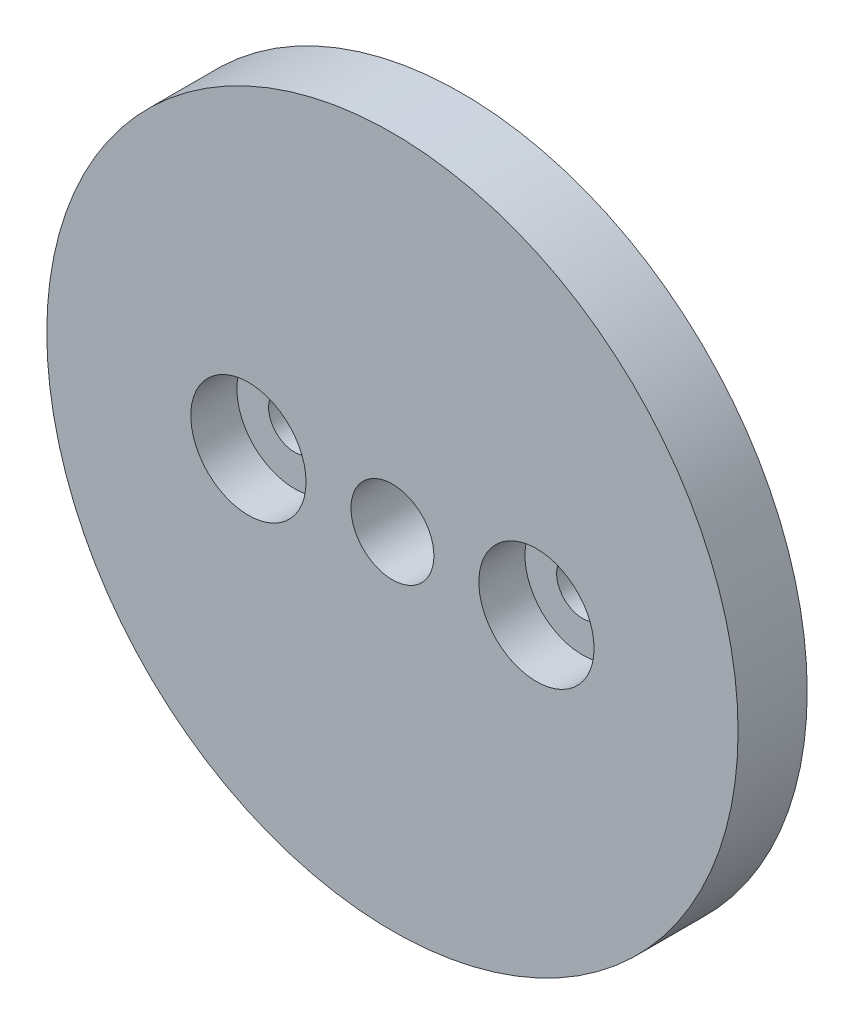
SolidWorks part; units mm, degrees
ref_plane "Front Plane" through (0, 0, 0) normal (0, 0, 1) x (1, 0, 0)
ref_plane "Top Plane" through (0, 0, 0) normal (0, 1, 0) x (1, 0, 0)
ref_plane "Right Plane" through (0, 0, 0) normal (1, 0, 0) x (0, 0, -1)
sketch "Sketch1" plane through (0, 0, 0) normal (0, 0, 1) x (1, 0, 0)
  circle A0 centre (0, 0) radius 30
  dimension "D1" = 60
extrude "Boss-Extrude1" add sketch "Sketch1" along normal blind 6
hole_wizard "CBORE for M4 Hex Head Bolt1" positions "Sketch2" profile "Sketch3" counterbore size "M4" standard "GB" end condition through all
sketch "Sketch2" plane through (0, 0, 6) normal (0, 0, 1) x (1, 0, 0)
  line L0 (0, 0) -> (0, 26.9917) construction
  point P0 (-12.5, 0)
  point P8 (12.5, 0)
  dimension "D1" = 12.5
sketch "Sketch3" plane through (-12.5, 0, 6) normal (1, 0, 0) x (0, -1, 0)
  line L0 (0, 0) -> (0, 6)
  line L1 (0, 6) -> (2.25, 6)
  line L3 (2.25, 6) -> (2.25, 4)
  line L4 (2.25, 4) -> (5, 4)
  line L5 (5, 4) -> (5, 0)
  line L7 (5, 0) -> (0, 0)
  line L11 (0, -6.35) -> (0, 107.95) construction
  dimension "通孔孔直径" = 4.5
  dimension "通孔孔深度" = 6
  dimension "柱形沉头孔直径" = 10
  dimension "柱形沉头孔深度" = 4
sketch "Sketch4" plane through (0, 0, 6) normal (0, 0, 1) x (1, 0, 0)
  circle A0 centre (0, 0) radius 3.6
  dimension "D1" = 7.2
extrude "Cut-Extrude1" cut sketch "Sketch4" against normal blind 10
